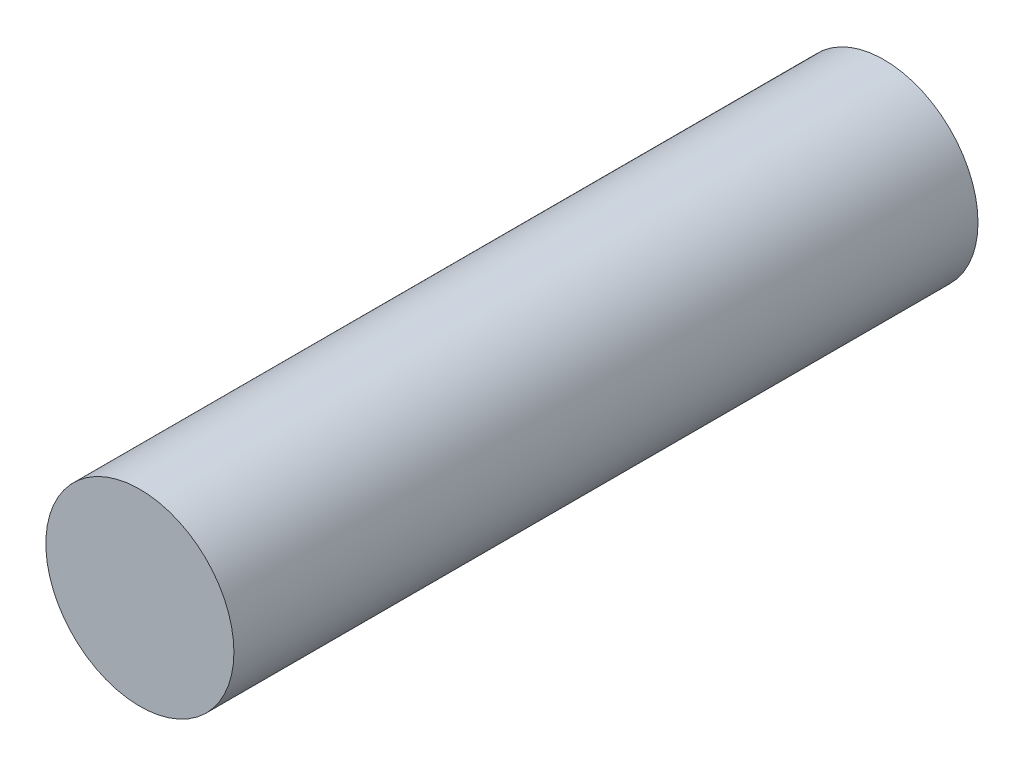
from build123d import *

# Parameters (mm, degrees)
SKETCH_1_R      = 1.15
EXTRUDE_1_DEPTH = 9.1


with BuildPart() as part:
    # 草图1 → 凸台-拉伸1 (new body)
    with BuildSketch(Plane.XY):
        Circle(SKETCH_1_R)
    extrude(amount=EXTRUDE_1_DEPTH)


solid = part.part
